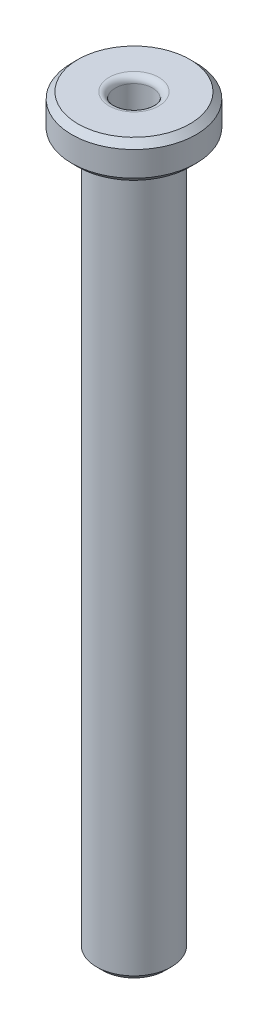
from build123d import *

# Parameters (mm, degrees)
SKETCH_1_R      = 3
SKETCH_1_R_2    = 1.5
EXTRUDE_1_DEPTH = 60
EXTRUDE_START   = -3
SKETCH_2_R      = 5
SKETCH_2_R_2    = 1.5
EXTRUDE_2_DEPTH = 3
FILLET_1_R      = 0.5
CHAMFER_1_SIZE  = 0.5


with BuildPart() as part:
    # 草图1 → 凸台-拉伸1 (new body)
    with BuildSketch(Plane(origin=(0, 0, 0), x_dir=(1, 0, 0), z_dir=(0, 1, 0))):
        with Locations(Location((0, 0, 0), (0, 0, 270))):
            Circle(SKETCH_1_R)
        with Locations(Location((0, 0, 0), (0, 0, 270))):
            Circle(SKETCH_1_R_2, mode=Mode.SUBTRACT)
    extrude(amount=EXTRUDE_1_DEPTH)

    # 草图2 → 凸台-拉伸2 (add)
    with BuildSketch(Plane(origin=(0, 60, 0), x_dir=(1, 0, 0), z_dir=(0, 1, 0)).offset(EXTRUDE_START)):
        with Locations(Location((0, 0, 0), (0, 0, 270))):
            Circle(SKETCH_2_R)
        with Locations(Location((0, 0, 0), (0, 0, 270))):
            Circle(SKETCH_2_R_2, mode=Mode.SUBTRACT)
    extrude(amount=EXTRUDE_2_DEPTH)

    # 圆角1
    fillet_1_edges = [part.edges().sort_by_distance(p)[0] for p in [
        (0, 0, -1.5),
        (0, 60, -1.5),
    ]]
    fillet(fillet_1_edges, radius=FILLET_1_R)

    # 倒角1
    chamfer_1_edges = [part.edges().sort_by_distance(p)[0] for p in [
        (0, 60, -5),
        (0, 57, -5),
        (0, 0, -3),
    ]]
    chamfer(chamfer_1_edges, length=CHAMFER_1_SIZE)


solid = part.part
